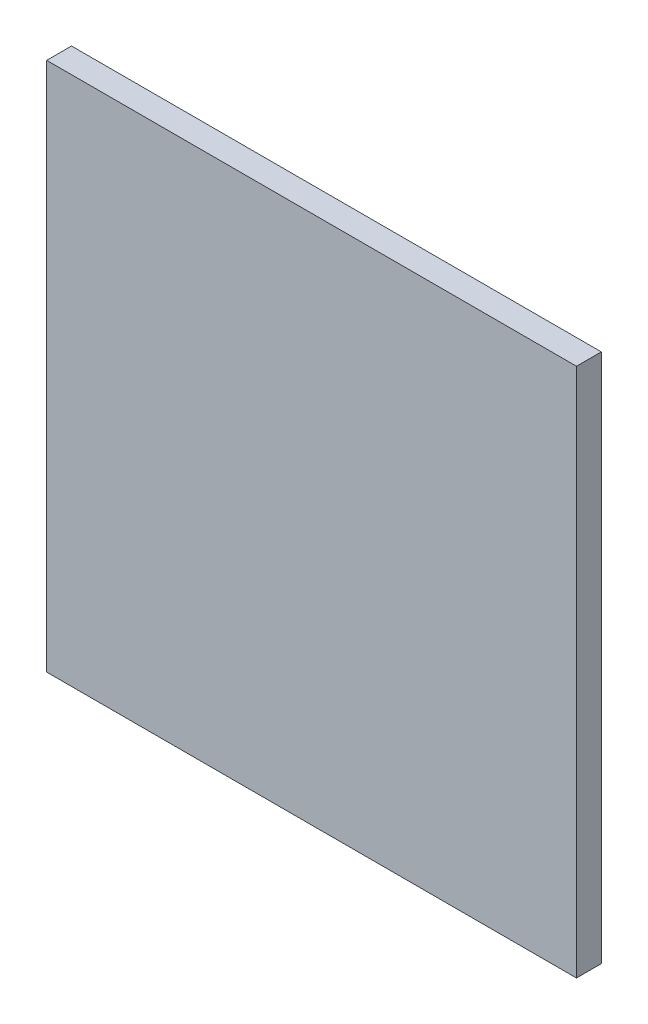
SolidWorks part; units mm, degrees
ref_plane "Front Plane" through (0, 0, 0) normal (0, 0, 1) x (1, 0, 0)
ref_plane "Top Plane" through (0, 0, 0) normal (0, 1, 0) x (1, 0, 0)
ref_plane "Right Plane" through (0, 0, 0) normal (1, 0, 0) x (0, 0, -1)
sketch "Sketch1" plane through (0, 0, 0) normal (0, 0, 1) x (1, 0, 0)
  line L1 (-16, 16) -> (16, 16)
  line L2 (-16, 16) -> (-16, -16)
  line L3 (-16, -16) -> (16, -16)
  line L4 (16, 16) -> (16, -16)
  line L5 (-16, 16) -> (16, -16) construction
  line L6 (-16, -16) -> (16, 16) construction
  point P0 (0, 0)
  dimension "D1" = 32
  dimension "D2" = 32
extrude "Boss-Extrude1" add sketch "Sketch1" along normal blind 1.5
